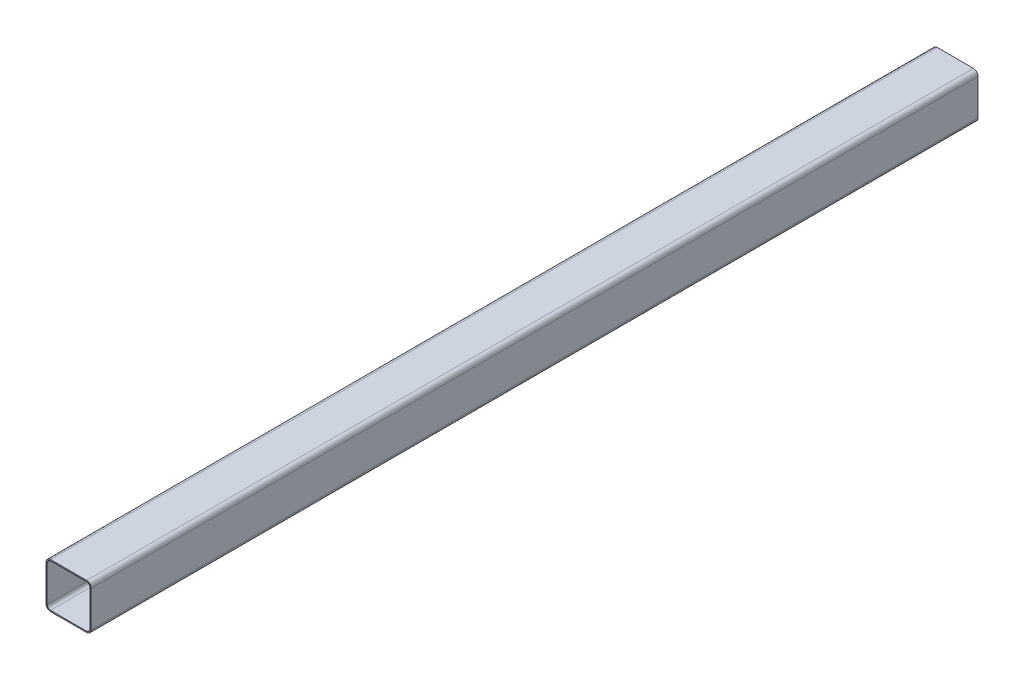
from build123d import *

# Parameters (mm, degrees)
BOSS_EXTRUDE1_DEPTH = 3930


with BuildPart() as part:
    # Sketch1 → Boss-Extrude1 (new body)
    with BuildSketch(Plane.XY):
        with BuildLine():
            Line((-80, 100), (80, 100))
            ThreePointArc((80, 100), (94.142135624, 94.142135624), (100, 80))
            Line((100, 80), (100, -80))
            ThreePointArc((100, -80), (94.142135624, -94.142135624), (80, -100))
            Line((80, -100), (-80, -100))
            ThreePointArc((-80, -100), (-94.142135624, -94.142135624), (-100, -80))
            Line((-100, -80), (-100, 80))
            ThreePointArc((-100, 80), (-94.142135624, 94.142135624), (-80, 100))
        make_face()
        with BuildLine():
            Line((-95, 80), (-95, -80))
            ThreePointArc((-95, -80), (-90.606601718, -90.606601718), (-80, -95))
            Line((-80, -95), (80, -95))
            ThreePointArc((80, -95), (90.606601718, -90.606601718), (95, -80))
            Line((95, -80), (95, 80))
            ThreePointArc((95, 80), (90.606601718, 90.606601718), (80, 95))
            Line((80, 95), (-80, 95))
            ThreePointArc((-80, 95), (-90.606601718, 90.606601718), (-95, 80))
        make_face(mode=Mode.SUBTRACT)
    extrude(amount=BOSS_EXTRUDE1_DEPTH)


solid = part.part
